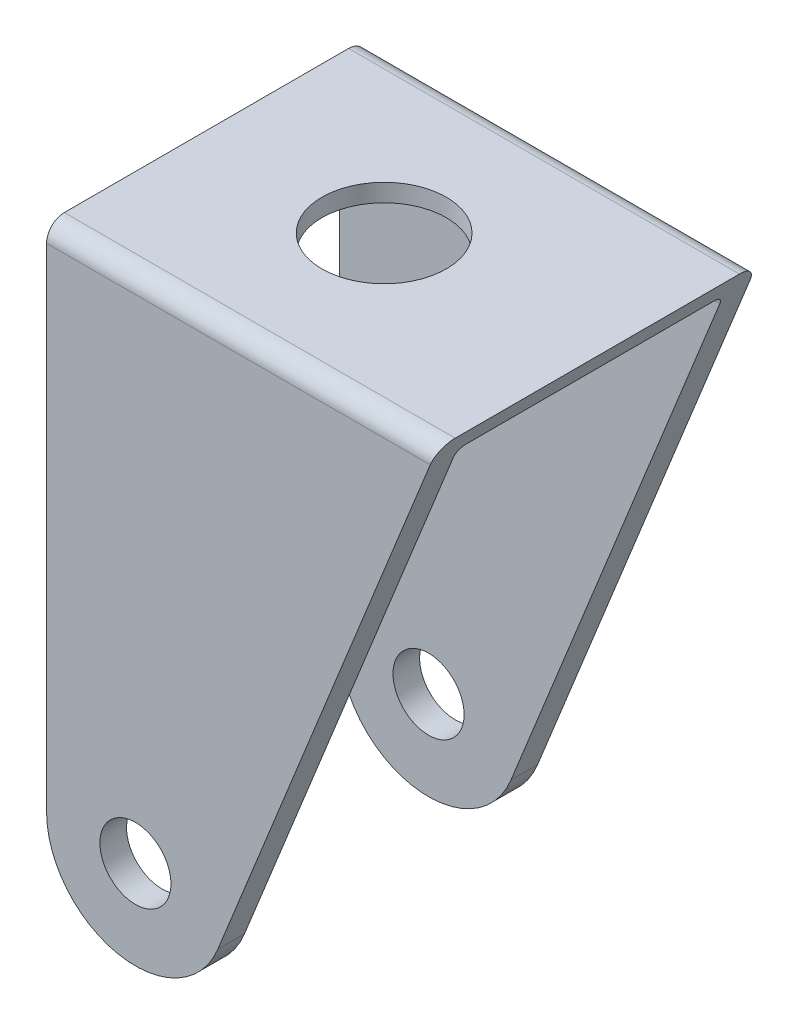
SolidWorks part; units mm, degrees
ref_plane "Front Plane" through (0, 0, 0) normal (0, 0, 1) x (1, 0, 0)
ref_plane "Top Plane" through (0, 0, 0) normal (0, 1, 0) x (1, 0, 0)
ref_plane "Right Plane" through (0, 0, 0) normal (1, 0, 0) x (0, 0, -1)
sketch "Sketch1" plane through (0, 0, 0) normal (0, 0, 1) x (1, 0, 0)
  line L0 (0, 0) -> (0, -57.4583)
  line L1 (0, 0) -> (44, 0)
  line L2 (44, 0) -> (19.2718, -61.2043)
  arc A0 (0, -57.4583) -> (19.2718, -61.2043) centre (10, -57.4583) ccw
  circle A1 centre (10, -57.4583) radius 4
  dimension "D3" = 10
  dimension "D4" = 8
  dimension "D1" = 44
  dimension "D2" = 22
extrude "Boss-Extrude1" add sketch "Sketch1" against normal blind 36
sketch "Sketch2" plane through (0, 0, 0) normal (-1, 0, 0) x (0, 0, 1)
  line L0 (-36, 0) -> (0, 0) construction
  line L1 (-36, 0) -> (0, 0) construction
  line L2 (-36, 0) -> (-36, -57.4583) construction
  line L3 (-36, 0) -> (-36, -57.4583) construction
  line L4 (-32, -2) -> (-4, -2)
  line L5 (-33, -3) -> (-33, -57.4583)
  line L6 (0, 0) -> (0, -57.4583) construction
  line L7 (0, 0) -> (0, -57.4583) construction
  line L8 (-3, -3) -> (-3, -57.4583)
  line L9 (-33, 0) -> (-33, -57.4583) construction
  line L10 (-36, -2) -> (0, -2) construction
  line L11 (-3, 0) -> (-3, -57.4583) construction
  line L13 (-3, -57.4583) -> (-3, -71.2844)
  line L14 (-3, -71.2844) -> (-33, -71.2844)
  line L15 (-33, -71.2844) -> (-33, -57.4583)
  arc A0 (-3, -3) -> (-4, -2) centre (-4, -3) ccw
  arc A1 (-33, -3) -> (-32, -2) centre (-32, -3) cw
  dimension "D4" = 1
  dimension "D5" = 13.8261
  dimension "D1" = 2
  dimension "D2" = 3
  dimension "D3" = 3
extrude "Cut-Extrude1" cut sketch "Sketch2" against normal blind 57
fillet "Fillet1" radius 2 2 edges at (22, 0, 0) (22, 0, -36)
sketch "Sketch3" plane through (0, 0, 0) normal (0, 1, 0) x (1, 0, 0)
  line L2 (0, 34) -> (0, 2) construction
  circle A0 centre (20, 18) radius 7
  dimension "D1" = 14
  dimension "D2" = 18
  dimension "D3" = 20
extrude "Cut-Extrude2" cut sketch "Sketch3" against normal blind 57
